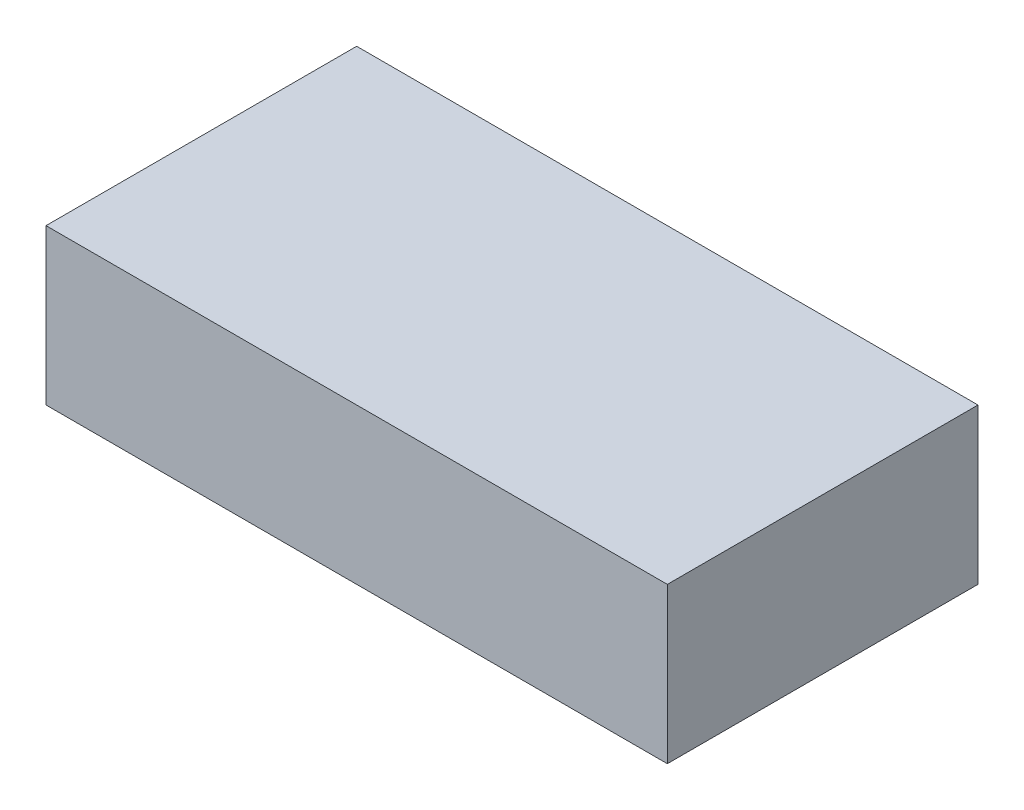
from build123d import *

# Parameters (mm, degrees)
SKETCH1_W           = 20
SKETCH1_H           = 10
BOSS_EXTRUDE1_DEPTH = 5


with BuildPart() as part:
    # Sketch1 → Boss-Extrude1 (new body)
    with BuildSketch(Plane(origin=(0, 0, 0), x_dir=(1, 0, 0), z_dir=(0, 1, 0))):
        Rectangle(SKETCH1_W, SKETCH1_H)
    extrude(amount=BOSS_EXTRUDE1_DEPTH)


solid = part.part
